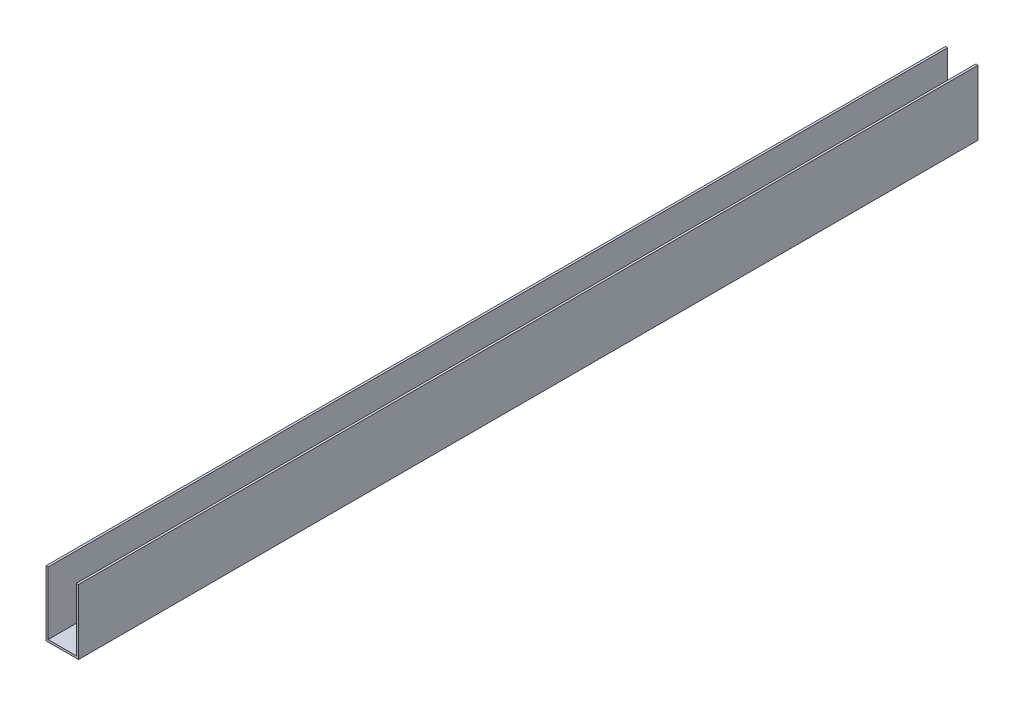
from build123d import *

# Parameters (mm, degrees)
SKETCH_1_W      = 30
SKETCH_1_H      = 60
EXTRUDE_1_DEPTH = 415
SHELL_1_T       = -2


with BuildPart() as part:
    # 草图1 → 凸台-拉伸1 (new, symmetric)
    with BuildSketch(Plane.XY):
        Rectangle(SKETCH_1_W, SKETCH_1_H)
    extrude(amount=EXTRUDE_1_DEPTH, both=True)

    # 抽壳1
    shell_1_openings = [part.faces().sort_by_distance(p)[0] for p in [
        (0, 0, 415),
        (0, 0, -415),
        (0, 30, 0),
    ]]
    offset(amount=SHELL_1_T, openings=shell_1_openings, kind=Kind.INTERSECTION)


solid = part.part
